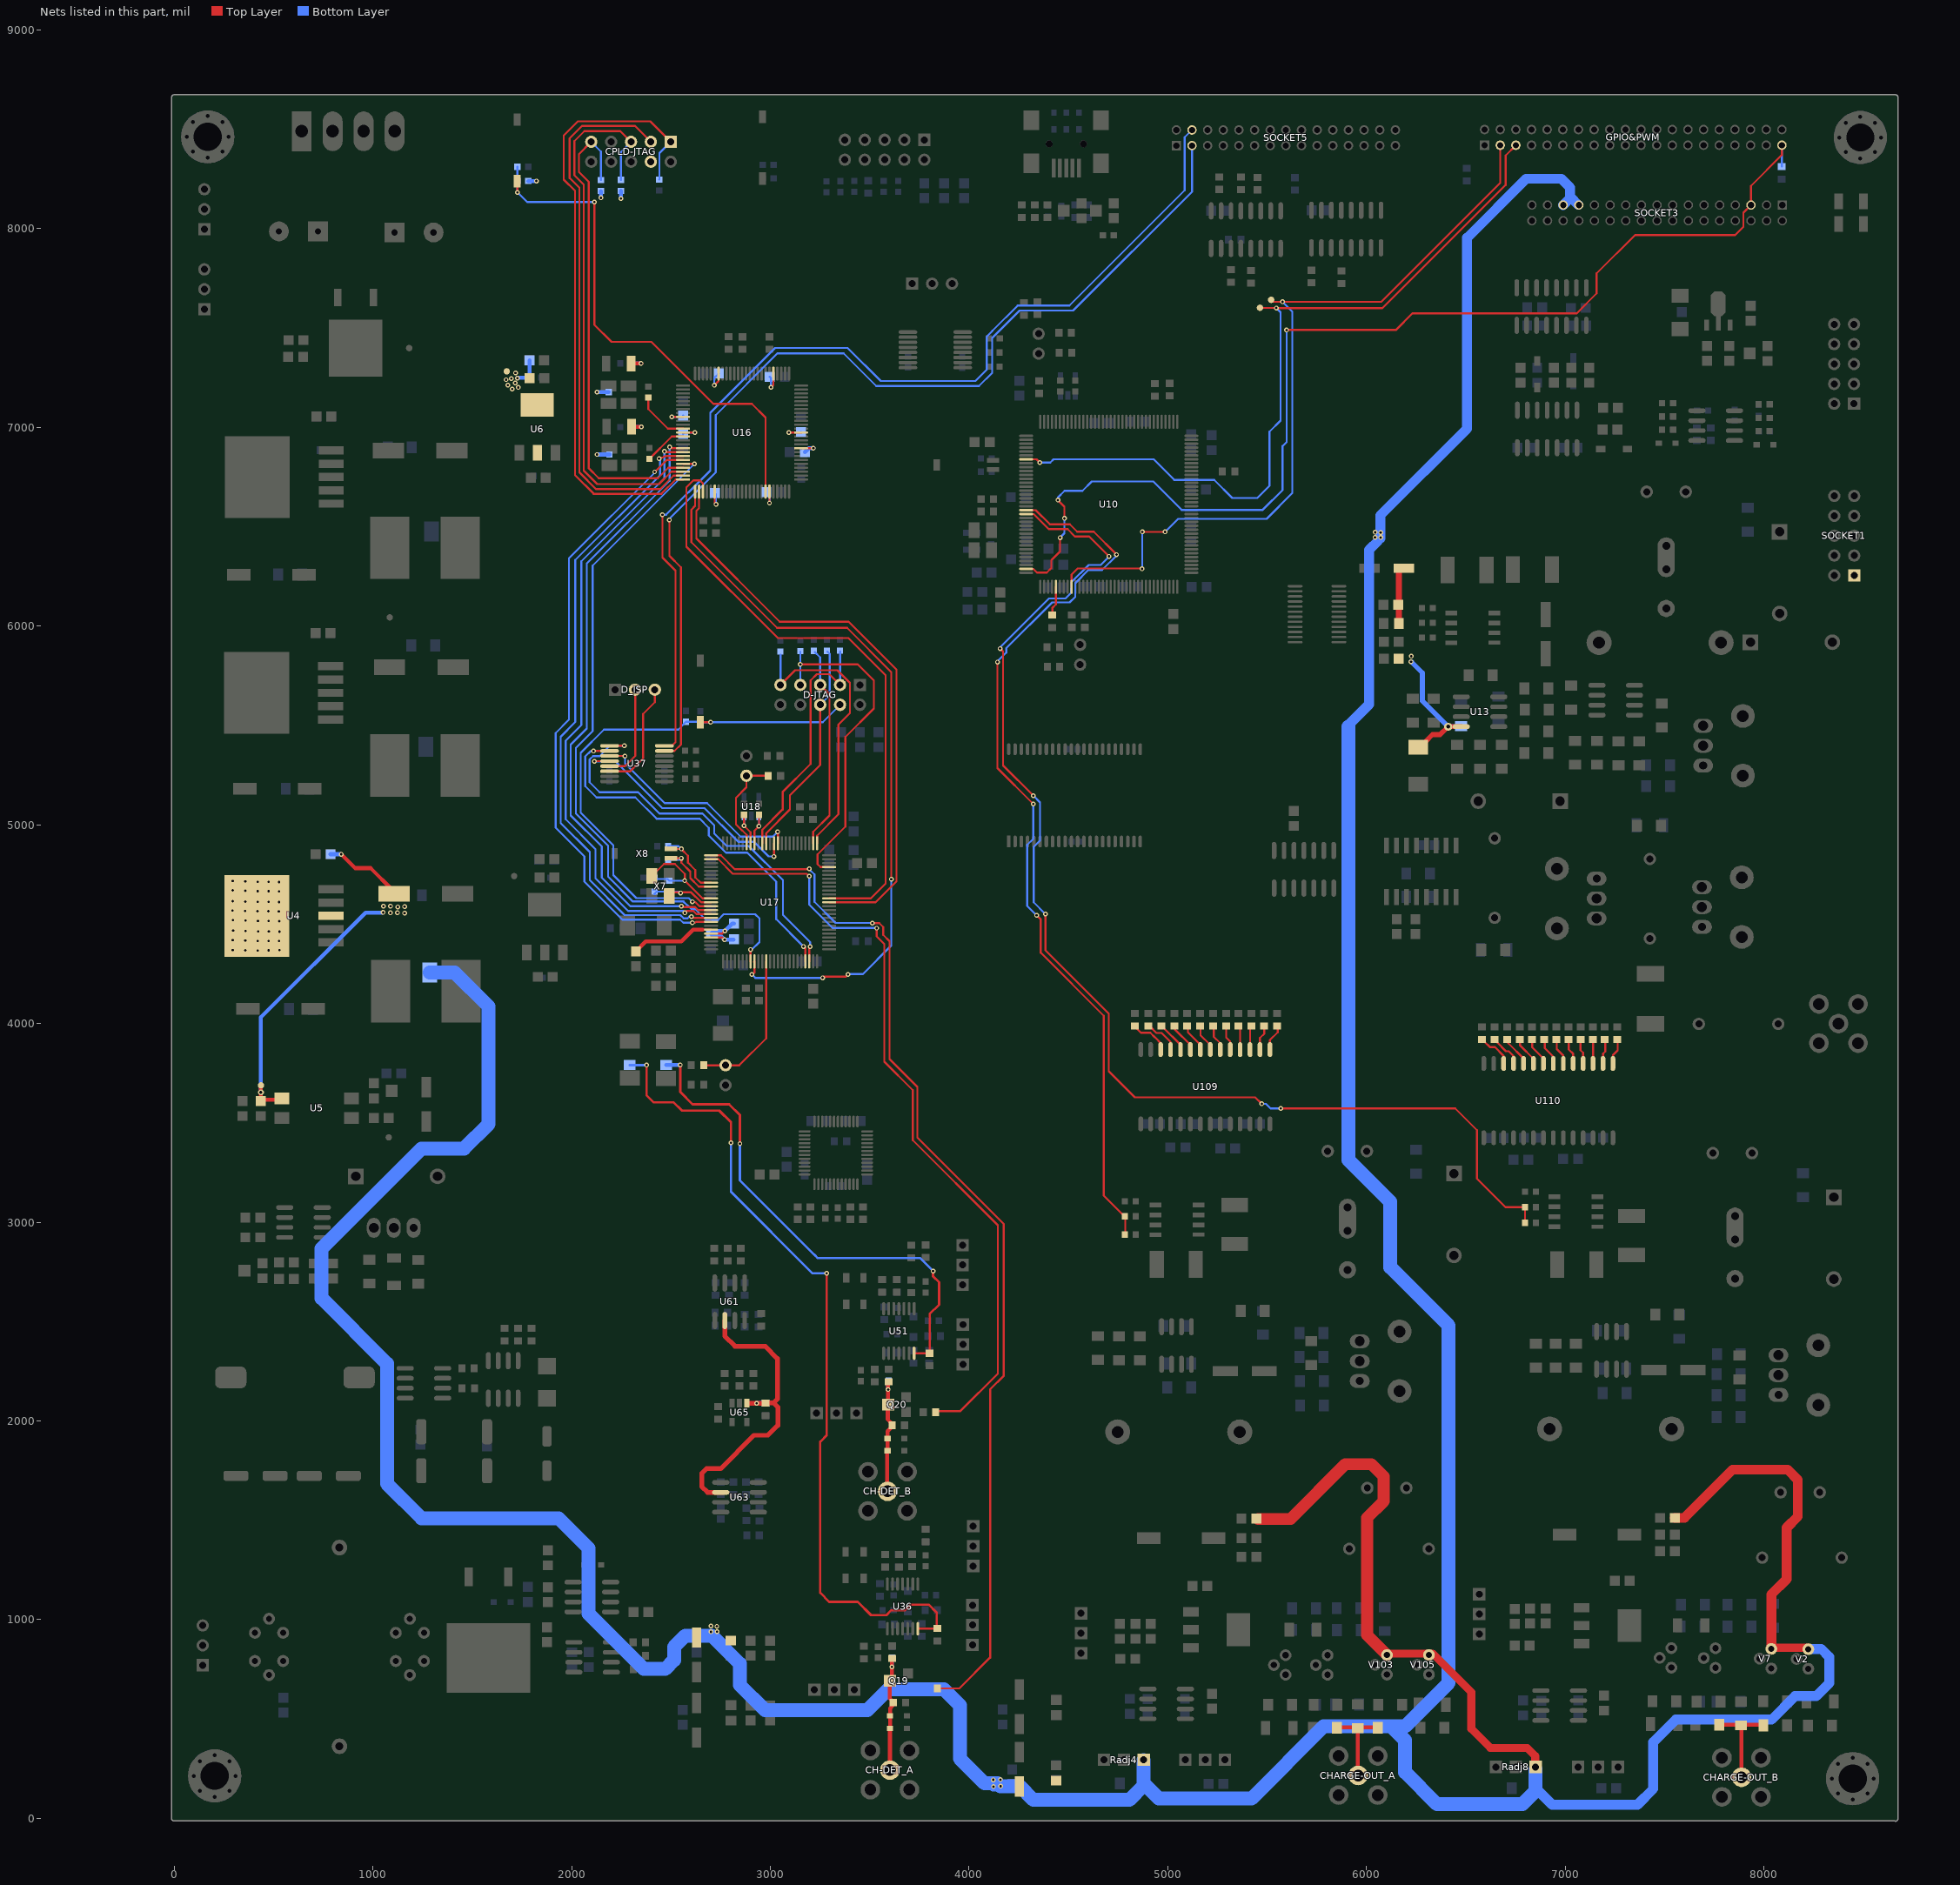
[diagram p0: the nets of this part, all layers, seen from the top]
# Altium PCB MISC82309.PcbDoc (part 5 of 14)
Units mil, origin at the board's own origin, x right, y up, seen from the top; angles counter-clockwise.
Board outline 8687.03 x 8687.86 mil, 4 copper layers (Top Layer, GND, POWER, Bottom Layer); 747 components, 583 nets, 2530 pads, 1834 vias.

## Via types
v1: diameter 24, hole 12, Top Layer to Bottom Layer, 1799 vias
v2: diameter 30, hole 15, Top Layer to Bottom Layer, 26 vias
v3: diameter 40, hole 20, Top Layer to Bottom Layer, 9 vias

## Nets (pads, with @x,y where several pads share a name; then routed paths per layer and width w, separated by ;. In a path a pad name is that pad's centre, name@x,y a point inside that pad or via, vN(x,y) a via of type N, cw(c..) or ccw(c..) an arc to the next point about the centre after c; other vN are vias at no path point) (continued)
-12V: C12.2 C13.2 C64.2 C65.2 C69.1 C156.1 C159.2 C174.2 C175.2 C278.1 D4.1 FB3.1 FB6.1 FB20.1 R4.1 R11.1 R45.1 R296.1 Radj4.3 Radj8.3 SOCKET3.27 SOCKET3.29 TP4.1 U4.3 U4.6 U5.3 V2.3 V7.3 V103.3 V105.3 | length 29056.6
  Top Layer w20: R11.1@437,3609.5 v2(437,3654) TP4.1@437,3689 ; R11.1@442,3616 U5.3@534.61,3616 ; v1(841,4852) 911,4782 989,4782 C12.2@1099,4672
  Top Layer w30: U5.3@534.61,3616 U5.3@542.8,3624.2 ; FB3.1@6163.39,6013 C64.2@6163.39,6286.61
  Top Layer w40: V103.3@6103,822.21 6110.32,829.53 6332.47,829.53 6527,635 6527,451 6623,355 6808,355 6849,314 Radj8.3@6849,266 ; Radj8.3@6850,263 Radj8.3@6850,266 ; V7.3@8037,853.21 8042.31,858.53 V2.3@8222.47,858.53
  Top Layer w50: R296.1@7551.5,1512 7599,1512 7842,1755 8119,1755 8170,1704 8170,1519 8114,1463 8114,1204 8037,1127 V7.3@8037,853.21
  Top Layer w60: R45.1@5455,1507 5618,1507 5894,1783 6024,1783 6086,1721 6086,1596 6003,1513 6003,922.21 V103.3@6103,822.21
  Bottom Layer w20: v2(437,3654) 437,4032 963,4558 v1@1049,4558 ; R4.1@787.5,4852 v1(841,4852) ; Radj4.3@4879,283 Radj4.3@4881,285 ; Radj8.3@6851,246 Radj8.3@6855,250
  Bottom Layer w50: v1@4122,161 v1@4159,161 ; Radj4.3@4881,285 Radj4.3@4881,296 ; 5917,5510 6013,5606 6013,6384 6059.5,6430.5 ; v1@6069,6471 6069,6557 6506,6994 6506,7954 6803,8251 6980,8251 7025,8206 7025,8154.36 SOCKET3.29@6989.64,8119 ; v1@6070,6441 v1@6070,6468 ; C278.1@6851,152 6934,69 7363,69 7443,149 7443,384 7556,497 8038,497 8156,615 8263,615 8329,681 8329,812 8288,853 V2.3@8232,853 ; Radj8.3@6851,246 Radj8.3@6851,259 Radj8.3@6851,263 ; 7030.64,8154.36 SOCKET3.27@7065,8120
  Bottom Layer w70: D4.1@1287,4257 1411,4257 1582,4086 1582,3494 1459,3371 1245,3371 742,2868 742,2618 1071,2289 1071,1684 1245,1510 1935,1510 2086,1359 2086,1030 2364,752 2471,752 2516,797 2516,863 2573,920 2705,920 2847,778 2847,671 2973,545 3489,545 3593,649 3874,649 3954,569 3954,301 4079,176 4143,176 ; v1(4159,162) 4255,162 4324,93 4806,93 4878,165 Radj4.3@4878,293 ; C69.1@4879,176 4955,100 5421,100 5784,463 6124,463 ; 5910,5493 5910,3313 6120,3103 6120,2773 6413,2480 6413,682 6194,463 6124,463 ; Radj8.3@6851,246 C278.1@6851,152 6851,138 6784,71 6355,71 6194,232 6194,393 6124,463
  other v1: 4123,160 4122,194 4158,195 2701,939 2732,940 2731,967 2701,968 421,4367 358,4368 475,4368 530,4369 295,4370 528,4415 421,4416 475,4416 358,4418 295,4420 530,4463 423,4464 477,4464 360,4466 297,4468 529,4515 422,4516 476,4516 359,4518 296,4520 1160,4556 1088,4557 1124,4558 1052,4559 527,4564 420,4565 474,4565 357,4567 294,4569 1125,4587 1160,4588 1089,4590 1053,4591 528,4611 421,4612 475,4612 358,4614 295,4616 528,4665 421,4666 475,4666 358,4668 295,4670 528,4712 421,4713 475,4713 358,4715 295,4717 6071,6446 6043,6447 6071,6471 6044,6472
-VCC: C423.1 C424.2 U61.6 U63.6 U65.1 | length 1590.4
  Top Layer w24: U63.6@2760,1641 2754,1641 U63.6@2750.51,1641 2684,1641 2654.5,1670.5 2654.5,1735.5 2679,1760 2750,1760 2918,1928 2988,1928 3038,1978 3038,2070 3018,2090 ; U61.6@2771,2505.51 2771,2427 2822,2376 2974,2376 3036,2314 3036,2110 3018,2092 3018,2090 ; U65.1@2882.4,2089.24 v1@2931.24,2089.24 ; v1(2931,2089) v1@2931.24,2089.24 ; C423.1@2978,2090 3018,2090 ; C423.1@2978,2091 2976.24,2089.24 v1@2931.24,2089.24
  Bottom Layer w24: v1(2931,2089) C424.2@2976,2089
AMP-12V: C53.1 D55.1 R91.2 U13.4 | length 672.8
  Top Layer w25: D55.1@6298,5420 6332,5454 6370,5454 6410,5494 v3(6411,5494) U13.4@6476.51,5494
  Bottom Layer w25: v1@6226,5820 6281,5765 6281,5624 v3(6411,5494) C53.1@6472,5494
  other v1: 6224,5821 6225,5848
ARM_PC5: GPIO&PWM.3 TP7.1 U10.45 | length 4034.9
  Top Layer w10: U10.45@4515.99,6197.65 4515.99,6258.99 4547,6290 4797,6290 ; 4803,6290 4797,6290 ; v1(4870,6288) 4868,6290 4797,6290 ; v1(4872,6474) v1(4986,6474) ; TP7.1@5520,7642 5530,7632 v1(5577,7632) 6074,7632 6672.74,8230.74 6672.74,8385 GPIO&PWM.3@6672.74,8420
  Bottom Layer w10: v1(4870,6288) 4872,6290 v1(4872,6474) ; v1(4986,6474) 5052,6540 5497,6540 5627,6670 5627,7582 v1(5577,7632)
ARM_PC8: GPIO&PWM.5 TP8.1 U10.7 | length 3976.5
  Top Layer w10: U10.7@4287.65,6839.38 4339.62,6839.38 v1(4356,6823) ; TP8.1@5473,7601 v1(5546,7601) 5547,7600 6080,7600 6700,8220 6700,8368.52 GPIO&PWM.5@6751.48,8420
  Bottom Layer w10: v1(4356,6823) 4408.62,6823 4425,6839.38 4929.62,6839.38 5033,6736 5234,6736 5325,6645 5450.94,6645 5512,6706.06 5512,6978 5568,7034 5568,7579 v1(5546,7601)
C_3V3: C20.2 C34.2 C75.2 C195.2 C196.2 C197.2 C198.2 C199.2 C200.2 C201.2 C202.2 C449.2 CPLD-JTAG.4 FB1.1 FB4.1 R16.1 R58.2 R100.1 R108.2 R232.2 R234.2 SOCKET1.1 TP6.1 U6.2 U6.4 U16.9 U16.13 U16.31 U16.45 U16.59 U16.63 U16.80 U16.94 | length 1540
  Top Layer w10: v1(2505,7053) 2506.48,7053 2506.74,7052.74 U16.9@2560.76,7052.74 ; U16.13@2560.76,6974 v1(2620,6974) ; v1(2718,7212) 2739.89,7233.89 U16.94@2739.89,7271.24 ; U16.31@2720.2,6676.76 2720.2,6619.8 v1(2727,6613) ; v1(2995.8,6619.8) U16.45@2995.8,6676.76 ; v1(3004,7202) 3015.48,7213.48 U16.80@3015.48,7271.24 ; v1(3093,6974) U16.63@3155.24,6974 ; U16.59@3155.24,6895.26 v1(3216.74,6895.26)
  Top Layer w20: FB1.1@2299.99,7322 v1(2350,7322) ; FB4.1@2301.99,7003 v1(2351,7003)
  Bottom Layer w10: v1@2512,7053 2554.5,7053 C199.2@2561,7059.5 ; C195.2@2561,6967.5 2567.5,6974 v1@2618,6974 ; v1@2718,7215 2718,7248.5 C197.2@2740.5,7271 ; C196.2@2720.5,6669 2726,6663.5 v1@2726,6616 ; v1@2996,6623 2996.5,6623.5 C200.2@2996.5,6676 ; C201.2@2997.5,7254 3004,7247.5 v1@3004,7206 ; v1@3095,6975 3151.5,6975 C202.2@3154,6977.5 ; C198.2@3154,6889.5 C198.2@3158.5,6894
  Bottom Layer w20: v1@1728,7249 1786,7249 1790,7253 1788.5,7254.5 R16.1@1788.5,7338 ; R100.1@1782.5,8240 v1(1823,8240) ; v1(2128.5,6863.5) R108.2@2191,6863.5 ; v1(2128.5,7177.5) R58.2@2187,7177.5 ; v1(2148,8155) R234.2@2148,8189.5 ; v1(2248,8152) R232.2@2248,8190.5 ; C34.2@2299.5,7322 v1@2347,7322 ; C75.2@2300.5,7002 2350,7002 v1(2351,7003) ; C198.2@3173.5,6876 3193.5,6896 v1@3217,6896
  other v1: 1701,7193 1732,7201 1679,7213 1717,7223 1671,7240 1697,7246 1727,7248 1718,7274
CH-DET_A: R199.2 R207.1 U36.7 | length 4187.7
  Top Layer w12: v1(2377,3791) 2377,3639 2412,3604 2513,3604 2555,3562 2743,3562 2802,3503 v1(2802,3400) ; v1(3284,2743) 3284,1929 3251,1896 3251,1135 3296,1090 3440,1090 3507,1023 3585,1023 3609.5,1047.5 3677.5,1047.5 3706,1076 3797,1076 3837,1036 R199.2@3837,961 ; U36.7@3742.77,954.8 3835.8,954.8 R199.2@3840,959
  Bottom Layer w12: R207.1@2292,3791 v1(2377,3791) ; v1@2802,3399 v1(2802,3400) 2802,3153 3212,2743 v1(3284,2743)
CH-DET_B: R110.1 R339.2 U51.7 | length 2580.3
  Top Layer w12: v1(2547,3792) 2547,3656 2609,3594 2793,3594 2847,3540 v1(2847,3395) ; U51.7@3723.77,2340.8 R339.2@3802,2340.8 ; R339.2@3802,2340.5 R339.2@3802,2340.8 ; R339.2@3807,2337 3803.2,2340.8 R339.2@3802,2340.8 ; v1(3819,2754) 3819,2728 3849,2698 3849,2585 3802,2538 R339.2@3802,2340.8
  Bottom Layer w12: v1(2847,3395) 2847,3351 2847,3211 3226,2832 ; 3223,2836 3239.5,2819.5 3754.5,2819.5 v1@3818,2756 ; v1@3816.5,2756.5 v1(3819,2754)
  Bottom Layer w20: R110.1@2476,3791 2477,3792 v1@2545,3792
CH-DETECT-IN_A: C165.2 CH-DET_A.1 D25.1 D26.2 Q19.3 R186.1 R545.2 | length 600.5
  Top Layer w20: CH-DET_A.1@3602,243 3602,436 3603,437 3603,555 3619,571 3619,586 3601,604 3601,672 Q19.3@3602,673 ; Q19.3@3602,692.5 3612,702.5 v1(3612,762) R186.1@3612,802
  Bottom Layer w20: v1@3612,767 3612,807.5 C165.2@3613,808.5
CH-DETECT-IN_B: C288.2 CH-DET_B.1 D46.2 D47.1 Q20.3 R322.1 R546.2 | length 601.9
  Top Layer w20: CH-DET_B.1@3587,1644 3588,1645 3588,1849 3589.68,1850.68 D47.1@3589.68,1912 3589.68,1948.68 3610,1969 3610,1988 3591,2007 Q20.3@3591,2064 ; Q20.3@3593,2082.5 3593,2196 R322.1@3597,2200
  Bottom Layer w20: v1(3593,2158) 3593,2200.5 C288.2@3595,2202.5
CH_A: R378.2 U17.1 | length 5378.3
  Top Layer w10: U17.1@2701.76,4846.22 2751.78,4846.22 2821,4777 3194,4777 v1(3196,4779) ; v1(3513,4505) 3548,4505 3568,4485 3568,4446 3600,4414 3600,3821 3740,3681 3740,3426 4175,2991 4175,2228 4106,2159 4106,809 3951,654 R378.2@3848,654
  Bottom Layer w10: v1(3196,4779) 3196,4775.94 3222,4749.94 3222,4612 3328,4506 3512,4506 v1(3513,4505)
CH_B: R379.2 U17.2 | length 3935.7
  Top Layer w10: U17.2@2701.76,4826.54 2738.46,4826.54 2811,4754 3183,4754 3195,4742 v1(3196,4742) ; v1(3535,4480) 3535,4439 3574,4400 3574,3808 3717,3665 3717,3413 4145,2985 4145,2238 3957,2050 R379.2@3843,2050
  Bottom Layer w10: v1(3196,4742) 3196,4598 3313,4481 3534,4481 v1(3535,4480)
CH_PHASE1: U16.17 U17.15 | length 3129.6
  Top Layer w10: v1(2493,6901) 2493,6900 2498,6895 2498.26,6895.26 U16.17@2560.76,6895.26 ; v1(2553,4590) 2553,4585 2554,4586 2621,4586 2636.37,4570.63 U17.15@2701.76,4570.63
  Bottom Layer w10: v1(2493,6901) 2493,6731 2077,6315 2077,5485 1996,5404 1996,5047 2152,4891 2152,4734 2296,4590 v1(2553,4590)
CH_PHASE2: U16.18 U17.16 | length 3156.2
  Top Layer w10: v1@2471.57,6875.57 U16.18@2560.76,6875.57 ; 2579,4566 2613,4566 2628.06,4550.94 U17.16@2701.76,4550.94
  Bottom Layer w10: v1(2467,6879) 2467,6744 2049,6326 2049,5502 1970,5423 1970,5028 2120.69,4877.31 2120.69,4730.31 2285,4566 2561,4566 v1(2570,4557)
CH_PHASE3: U16.19 U17.17 | length 3186.1
  Top Layer w10: v1(2440,6843) 2438,6843 2437,6844 2441,6848 2460.96,6848 2467.96,6855 2476.94,6855 ; 2477.83,6855.89 U16.19@2560.76,6855.89 ; v1@2612.74,4531.26 U17.17@2701.76,4531.26
  Bottom Layer w10: v1@2445,6836 2445,6759 2019,6333 2019,5517 1945,5443 1945,5009 2091.5,4862.5 2091.5,4721.5 2266.97,4546.03 2547.03,4546.03 2564.06,4529 2583,4529 v1@2592,4538
  other v1: 2603,4538
CH_PHASE4: U16.20 U17.18 | length 3209.2
  Top Layer w10: v1@2419,6776 2479.2,6836.2 U16.20@2560.76,6836.2 ; 2622,4507 2626.57,4511.57 U17.18@2701.76,4511.57
  Bottom Layer w10: v1@2423.5,6777.5 1987,6341 1987,5529 1920,5462 1920,4986 2065,4841 2065,4714 2256,4523 2546.02,4523 2562.02,4507 v1(2608,4507)
  other v1: 2418,6776
CH_PHASE5: U16.21 U17.33 | length 3562.8
  Top Layer w10: U16.21@2560.76,6816.52 v1(2618.48,6816.52) ; U17.33@2900.57,4312.76 v1(2900.57,4372.57) ; U17.33@2901.48,4312.76 U17.33@2901.48,4318.02
  Bottom Layer w10: 2581.94,4595 2562.94,4614 2309,4614 2184,4739 2184,4895 2022,5057 2022,5387 2106.5,5471.5 2106.5,6304.5 2618,6816 v1@2618.48,6816 ; 2584,4595 2604,4575 2623,4575 2677,4521 2736,4521 2765,4550 2924,4550 2945,4529 2945,4410.52 2907.05,4372.57 v1(2900.57,4372.57)
CH_PHASE6: U16.26 U17.34 | length 3745.1
  Top Layer w10: U16.26@2621.78,6676.76 2621.78,6604.78 2603,6586 2603,6422 3034,5991 3386,5991 3609,5768 v1(3609,4726) ; v1@2913,4249 2920.26,4256.26 U17.34@2920.26,4312.76 U17.34@2918.48,4310.98 ; v1@3269,4236 3380,4236 v1(3391,4247)
  Bottom Layer w10: v1@2914,4246 2914,4241 2925,4230 v1(3263,4230) ; v1@3393,4249 3466,4249 3609,4392 v1(3609,4726)
  other v1: 2907,4247
CH_PHASE7: U16.27 U17.63 | length 2970
  Top Layer w10: U16.27@2641.46,6676.76 2641.46,6593.46 2628,6580 2628,6441 3047,6022 3394,6022 3635,5781 3635,4715 3530,4610 U17.63@3296.24,4610
CH_PHASE8: U16.28 U17.64 | length 3076.6
  Top Layer w10: U16.28@2661.15,6676.76 2661.15,6718 2646.15,6733 2613,6733 2578,6698 2578,6400 3038,5940 3393,5940 3580,5753 3580,4704 3505.68,4629.68 U17.64@3296.24,4629.68
CHARGE-CTRL_A: R151.2 R312.2 U10.20 | length 4596.2
  Top Layer w10: v1(4143,5819) 4143,5285 v1(4323,5105) ; U10.20@4287.65,6583.47 4335.53,6583.47 4407,6512 4507,6512 4544,6475 4628,6475 v1@4742.5,6360.5 ; v1(4340,4545) 4361,4524 4361,4356 4678,4039 4678,3134 4786,3026 R151.2@4786,2939
  Bottom Layer w10: v1@4143,5823 4187,5867 4187,5888 4418,6119 4506,6119 4534,6147 4534,6216 4600,6282 4668.94,6282 4742,6355.06 v1(4742,6360) v1@4741.5,6359.5 ; v1(4323,5105) 4323,4929 4293,4899 4293,4592 v1(4340,4545)
CHARGE-CTRL_B: R343.2 R344.2 U10.21 | length 6265.2
  Top Layer w10: v1(4156,5887) 4171,5872 4171,5299 v1(4323,5147) ; U10.21@4287.65,6563.79 4325.21,6563.79 4401,6488 4495.79,6488 4532.79,6451 4604,6451 v1(4704,6351) ; v1(4384,4551) 4384,4369 4703,4050 4703,3760 4834,3629 5440,3629 v1(5473,3596) ; v1(5569,3573) 6446,3573 6556,3463 6556,3219 6699,3076 R344.2@6797,3076 ; R344.2@6796,3077 R344.2@6797,3076 ; R343.2@6797.5,2997 6797.5,3075.5 R344.2@6797,3076 ; R344.2@6797.5,3076 R344.2@6797,3076
  Bottom Layer w10: v1(4156,5887) 4153,5890 4402,6139 4485,6139 4514,6168 4514,6220.04 4601.96,6308 4663,6308 v1@4704,6349 ; v1(4323,5147) 4357,5113 4357,4921 4325,4889 4325,4610 v1(4384,4551) ; v1(4704,6351) v1@4704,6349 ; v1@4705,6350 v1@4704,6349 ; v1(5473,3596) 5494,3596 5517,3573 v1(5569,3573)
CHARGE_OUT_A: CHARGE-OUT_A.1 R152.1 R202.2 R203.2 | length 426.1
  Top Layer w20: R203.2@5852,461 5854,459 6054,459 R152.1@6057,456 ; CHARGE-OUT_A.1@5956,235 R202.2@5956,454
CHARGE_OUT_B: CHARGE-OUT_B.1 R302.2 R303.2 R304.1 | length 478
  Top Layer w20: R303.2@7774,472 R304.1@7997,472 ; CHARGE-OUT_B.1@7887,207 R302.2@7887,462
CLK0: R59.1 U16.12 | length 274
  Top Layer w10: R59.1@2386,7150.5 2386,7092 2484.32,6993.68 U16.12@2560.76,6993.68
CLK1: R109.1 U16.14 | length 215.5
  Top Layer w10: R109.1@2392,6841.5 2504.81,6954.31 U16.14@2560.76,6954.31
COUNT-RESET: GPIO&PWM.39 R404.2 SOCKET3.5 U10.35 | length 5789.4
  Top Layer w10: U10.35@4287.65,6288.2 4322.81,6288.2 4342.01,6269 4391,6269 4414,6292 4414,6332 4458,6376 v1(4458,6445) ; v1(4447,6634) 4480,6601 v1(4480,6542) ; v1(5598,7490) 6147,7490 6231,7574 7058,7574 7158,7674 7158,7775 7351,7968 7855,7968 7896,8009 7896,8080.48 SOCKET3.5@7934.52,8119 7934.52,8215.52 8090.06,8371.06 GPIO&PWM.39@8090.06,8420
  Bottom Layer w10: v1(4447,6634) 4447,6647 4481,6681 4571,6681 4618,6728 4927,6728 5070,6585 5478,6585 5578,6685 5578,6906 5598,6926 v1(5598,7490) ; v1(4458,6445) 4480,6467 v1(4480,6542) ; R404.2@8090,8312.5 8090,8419.94 GPIO&PWM.39@8090.06,8420
CPLD_RST: C244.2 CPLD_REST.2 R100.2 U16.44 | length 2635.1
  Top Layer w10: CPLD_REST.2@1727,8239 1727,8183 v1(1727.5,8182.5) ; v1(2115,8134) 2115,7516 2201,7430 2402,7430 2713.94,7118.06 2907.06,7118.06 2976.11,7049 U16.44@2976.11,6676.76
  Bottom Layer w10: v1@1727.5,8176.5 1734.5,8176.5 1777,8134 v1(2115,8134) ; v1(1727.5,8182.5) R100.2@1727.5,8240 C244.2@1727.5,8311
CPLD_TCK: CPLD-JTAG.1 R294.2 U16.25 | length 3169.2
  Top Layer w10: CPLD-JTAG.1@2499,8437 2396,8540 2032,8540 1961,8469 1961,8247 2017,8191 2017,6760 2111,6666 2452,6666 2523.78,6737.78 U16.25@2560.76,6737.78
  Bottom Layer w10: R294.2@2441,8246.5 2442,8247.5 2442,8380 CPLD-JTAG.1@2499,8437
CPLD_TDI: CPLD-JTAG.9 R234.1 U16.22 | length 2418.5
  Top Layer w10: CPLD-JTAG.9@2099,8437 2037,8375 2037,8285 2087,8235 2087,6794 2137,6744 2434,6744 2486.83,6796.83 U16.22@2560.76,6796.83
  Bottom Layer w10: CPLD-JTAG.9@2099,8437 2148,8388 R234.1@2148,8244.5
CPLD_TDO: CPLD-JTAG.3 U16.24 | length 2753.6
  Top Layer w10: CPLD-JTAG.3@2399,8437 2319,8517 2052,8517 1990,8455 1990,8255 2039,8206 2039,6774 2123,6690 2446,6690 2513.46,6757.46 U16.24@2560.76,6757.46
CPLD_TMS: CPLD-JTAG.5 R232.1 U16.23 | length 2771.8
  Top Layer w10: CPLD-JTAG.5@2299,8437 2245,8491 2064,8491 2014,8441 2014,8269 2061,8222 2061,6783 2129,6715 2440,6715 2502.15,6777.15 U16.23@2560.76,6777.15
  Bottom Layer w10: R232.1@2248,8245.5 2248,8386 CPLD-JTAG.5@2299,8437
D_A0: R547.1 U109.12 | length 190.3
  Top Layer w10: R547.1@4840,3979 4865.5,3953.5 4912.5,3953.5 4935,3931 4939,3927 U109.12@4964,3902 ; U109.12@4964,3869.01 U109.12@4964,3902 ; U109.12@4965,3901 U109.12@4964,3902
D_A1: R548.1 U109.11 | length 175.9
  Top Layer w10: R548.1@4911,3985 4943,3953 4969,3953 5014,3908 U109.11@5014,3869.01 ; R548.1@4912,3979 R548.1@4912,3981
D_A2: R549.1 U109.10 | length 147
  Top Layer w10: R549.1@4977,3980 5064,3893 U109.10@5064,3869.01
D_A3: R550.1 U109.9 | length 155.3
  Top Layer w10: R550.1@5036,3992 5036,3970 5114,3892 U109.9@5114,3869.01
D_A4: R525.1 U109.8 | length 140.1
  Top Layer w10: R525.1@5101,3983 5101,3956 5164,3893 U109.8@5164,3869.01
D_A5: R526.1 U109.7 | length 134.3
  Top Layer w10: R526.1@5165,3983 5165,3941 5214,3892 U109.7@5214,3869.01
D_A6: R527.1 U109.6 | length 131.7
  Top Layer w10: R527.1@5231,3987 5231,3934 5264,3901 U109.6@5264,3869.01
D_A7: R528.1 U109.5 | length 125.3
  Top Layer w10: R528.1@5294,3986 5294,3930 5314,3910 U109.5@5314,3869.01
D_A8: R529.1 U109.4 | length 118.1
  Top Layer w10: R529.1@5359,3985 5364,3980 U109.4@5364,3869.01
D_A9: R530.1 U109.3 | length 117.4
  Top Layer w10: R530.1@5413,3986 5414,3985 U109.3@5414,3869.01
D_A10: R531.1 U109.2 | length 127.1
  Top Layer w10: U109.2@5464,3869.01 5464,3927 5486,3949 R531.1@5486,3987
D_A11: R532.1 U109.1 | length 134.1
  Top Layer w10: U109.1@5514,3869.01 5514,3917 5553,3956 R532.1@5553,3987
D_AGND: R222.1 U17.20 | length 433.1
  Top Layer w11: 2649.2,4472.2 2659.52,4472.2 U17.20@2701.76,4472.2
  Top Layer w20: R222.1@2324,4363.5 2373.5,4413 2552,4413 2611.2,4472.2 2659.52,4472.2
D_B0: R533.1 U110.12 | length 170.8
  Top Layer w10: R533.1@6593,3913 6593,3909 6620,3882 6645,3882 6690,3837 U110.12@6690,3799.01 U110.12@6690,3801
D_B1: R534.1 U110.11 | length 152
  Top Layer w10: R534.1@6656,3908 6656,3906 6701,3861 6715,3861 6740,3836 U110.11@6740,3799.01
D_B2: R535.1 U110.10 | length 157.4
  Top Layer w10: R535.1@6713,3922 6713,3901 6793,3821 6793,3802.01 U110.10@6790,3799.01
D_B3: R536.1 U110.9 | length 140.7
  Top Layer w10: R536.1@6773,3912 6773,3889 6840,3822 U110.9@6840,3799.01
D_B4: R537.1 U110.8 | length 142.2
  Top Layer w10: R537.1@6834,3918 6834,3880 6890,3824 U110.8@6890,3799.01
D_B5: R538.1 U110.7 | length 136.8
  Top Layer w10: R538.1@6897,3918 6897,3876 6940,3833 U110.7@6940,3799.01
D_B6: R539.1 U110.6 | length 128.7
  Top Layer w10: R539.1@6957,3914 6957,3872 6990,3839 U110.6@6990,3799.01
D_B7: R540.1 U110.5 | length 127.5
  Top Layer w10: R540.1@7017,3917 7017,3870 7040,3847 U110.5@7040,3799.01
D_B8: R541.1 U110.4 | length 122.4
  Top Layer w10: R541.1@7077,3916 7077,3866 7090,3853 U110.4@7090,3799.01
D_B9: R542.1 U110.3 | length 121.4
  Top Layer w10: R542.1@7139,3920 7140,3919 U110.3@7140,3799.01
D_B10: R543.1 U110.2 | length 121.5
  Top Layer w10: U110.2@7190,3799.01 7190,3848 7201,3859 R543.1@7201,3916
D_B11: R544.1 U110.1 | length 123.9
  Top Layer w10: U110.1@7240,3799.01 7240,3841 7264,3865 R544.1@7264,3913
D_BOOT0: D_BOOT0.2 R61.1 U17.94 | length 493.1
  Top Layer w10: U17.94@2880.89,4907.24 2880.89,4949.11 2859,4971 2858.06,4971 2827,5002.06 2827,5136 2880,5189 D_BOOT0.2@2880,5247 R61.1@2988.5,5247
D_BOOT1: D_BOOT1.2 R62.1 U17.37 | length 757.7
  Top Layer w10: R62.1@2665.5,3791 2666.5,3790 D_BOOT1.2@2775,3790 2844,3790 2979.32,3925.32 U17.37@2979.32,4312.76
D_ISP_RX: D_ISP.2 U37.13 | length 485.1
  Top Layer w10: U37.13@2191.2,5295.2 2269.2,5295.2 2321,5347 2321,5678 D_ISP.2@2319,5680
D_ISP_TX: D_ISP.3 U37.14 | length 565.9
  Top Layer w10: U37.14@2191.2,5269.61 2295.61,5269.61 2360,5334 2360,5558 2419,5617 D_ISP.3@2419,5680
D_JNTRST: D-JTAG.3 R592.1 U17.90 | length 1273.6
  Top Layer w10: U17.90@2959.63,4907.24 2959.63,4974.63 3062,5077 3062,5098 3062,5165 3203,5306 3203,5727 3234,5758 3297,5758 D-JTAG.3@3351,5704
  Bottom Layer w10: D-JTAG.3@3351,5704 3351,5871 R592.1@3353,5873
D_JTCK: D-JTAG.9 R595.2 U17.76 | length 1436.1
  Top Layer w10: D-JTAG.9@3051,5704 3125,5778 3232,5778 3337.81,5778 3401,5714.81 3401,5562 3343,5504 3343,5053 3235.22,4945.22 U17.76@3235.22,4907.24
  Bottom Layer w10: D-JTAG.9@3051,5704 R595.2@3051,5857
D_JTDI: D-JTAG.5 R593.1 U17.77 | length 1028
  Top Layer w10: U17.77@3215.54,4907.24 3215.54,4964.54 3298,5047 3298,5657 D-JTAG.5@3251,5704
  Bottom Layer w10: R593.1@3223,5870 3251,5842 D-JTAG.5@3251,5704
D_JTDO: D-JTAG.6 R596.2 U17.89 | length 1100.7
  Top Layer w10: U17.89@2979.32,4907.24 2979.32,4957.32 3099,5077 3099,5102 3099,5149 3251,5301 D-JTAG.6@3251,5604
  Bottom Layer w10: D-JTAG.6@3251,5604 3299,5652 3299,5860 R596.2@3288,5871
D_JTMS: D-JTAG.7 R594.1 U17.72 | length 1692.6
  Top Layer w10: v1(3151,5808) 3439,5808 3521,5726 3521,5585 3378,5442 3378,4991 3238,4851 3238,4802 3252.83,4787.17 U17.72@3296.24,4787.17
  Bottom Layer w10: D-JTAG.7@3151,5704 3151,5773 ; 3151,5788 3151,5773 ; R594.1@3151,5872 v1(3151,5808) 3151,5773
D_NRST: C74.2 D-JTAG.4 D_REST.1 R113.2 U17.14 | length 2697.2
  Top Layer w10: v1@2608,4611 2623,4611 2643.68,4590.32 U17.14@2701.76,4590.32 ; D_REST.1@2648,5516 v1@2699.5,5516
  Bottom Layer w10: v1(2608,4613) 2590,4631 2326,4631 2210,4747 2210,4897 2046,5061 2046,5362 2163.25,5479.25 2536.75,5479.25 C74.2@2576,5518.5 2646,5518.5 R113.2@2648,5516.5 v1(2700,5516.5) 3263.5,5516.5 D-JTAG.4@3351,5604
D_OSC32_IN: C84.2 U17.8 X8.1 | length 385.5
  Top Layer w10: X8.1@2500,4878.62 v1(2553,4878.62) v1@2554,4878.62 ; v1@2554,4876 2585.5,4844.5 ; 2585,4844 2585,4810 2623,4772 2623,4735 2649.57,4708.43 U17.8@2701.76,4708.43
  Bottom Layer w10: C84.2@2486.5,4893 2538.62,4893 v1(2553,4878.62)
D_OSC32_OUT: C85.2 U17.9 X8.4 | length 365.1
  Top Layer w10: X8.4@2502.38,4829 X8.4@2500,4831.38 v1@2553,4831.38 ; v1@2553,4831 2553,4809 2597,4765 2597,4732 2640.26,4688.74 U17.9@2701.76,4688.74
  Bottom Layer w10: C85.2@2486.5,4824 2544,4824 v1(2552,4832)
D_OSC_IN: C80.2 R114.1 U17.12 X7.1 | length 571.2
  Top Layer w10: X7.1@2404,4742 2465,4803 2520,4803 2570,4753 2570,4719 2659.32,4629.68 U17.12@2701.76,4629.68
  Bottom Layer w10: C80.2@2415.5,4727 2482.5,4727 R114.1@2491,4718.5 v1@2568.5,4718.5
  other v1: 2569,4719
D_OSC_OUT: C81.2 R114.2 U17.13 X7.3 | length 380.7
  Top Layer w10: X7.3@2490.61,4642 2508.61,4660 2602,4660 2652,4610 U17.13@2701.76,4610
  Bottom Layer w10: C81.2@2415.5,4651 2428,4663.5 2542.5,4663.5 v1(2549,4657)
D_OUT: R558.1 U10.41 | length 140.2
  Top Layer w10: R558.1@4419,6065 4419,6091 4437.25,6109.25 U10.41@4437.25,6197.65
D_RS232_RXD: SOCKET5.4 U37.8 | length 5264.8
  Top Layer w10: v1(2457,6560) 2457,6345 2523,6279 2523,5416 2504.57,5397.57 U37.8@2466.8,5397.57
  Bottom Layer w10: v1@2457,6561 2476,6561 2698,6783 2698,7074 3024,7400 3389,7400 3556,7233 4032,7233 4089,7290 4089,7457 4114,7482 4118,7486 4245,7613 4505,7613 5085,8193 5085,8460 SOCKET5.4@5121.74,8496.74
D_RS232_TXD: SOCKET5.3 U37.7 | length 5201.4
  Top Layer w10: U37.7@2466.8,5371.98 2517.98,5371.98 2550,5404 2550,6296 2492,6354 v1@2492,6528
  Bottom Layer w10: v1@2492,6535 2492,6541 2725,6774 2725,7062 3035,7372 3369,7372 3533,7208 4050,7208 4116,7274 4116,7450 4254,7588 4524,7588 5121.74,8185.74 SOCKET5.3@5121.74,8418
  other v1: 2492,6534
D_SCL: R111.2 U17.92 U18.1 | length 204.7
  Top Layer w10: U17.92@2920.26,4907.24 2920.26,4970.26 v1(2943,4993) R111.2@2943,5050.5
  Bottom Layer w10: U18.1@2942.4,5044.76 2943,5044.16 v1(2943,4993)
D_SDA: R112.2 U17.93 U18.3 | length 206.7
  Top Layer w10: R112.2@2868,5050.5 v1(2868,4995) 2900.57,4962.43 U17.93@2900.57,4907.24
  Bottom Layer w10: U18.3@2867.6,5044.76 2867.6,4995.4 v1(2868,4995)
D_USART2_RX: U17.87 U37.12 | length 1244.5
  Top Layer w10: v1(2115,5319) 2116.8,5320.8 U37.12@2191.2,5320.8 ; v1(3018,4841) 3018.68,4841.68 U17.87@3018.68,4907.24
  Bottom Layer w10: v1(2115,5319) 2221,5319 2456,5084 2669,5084 2838,4915 2917,4915 2991,4841 v1(3018,4841)
D_USART2_TX: U17.86 U37.11 | length 1104.2
  Top Layer w10: U37.11@2191.2,5346.39 2268.61,5346.39 v1(2269,5346) ; v1(3037,4965) 3038.37,4963.63 U17.86@3038.37,4907.24
  Bottom Layer w10: v1(2269,5346) 2269,5308 2468,5109 2682,5109 2850,4941 3013,4941 v1(3037,4965)
D_USART3_RX: U17.48 U37.9 | length 2060.5
  Top Layer w10: U37.9@2191.2,5397.57 2264.57,5397.57 v1(2265,5398) ; U17.48@3195.85,4312.76 3195.85,4381.85 v1(3201,4387)
  Bottom Layer w10: v1(2265,5398) 2193,5398 2141,5346 2108.06,5346 2091,5328.94 2091,5214 2141,5164 2335,5164 2442,5057 2659,5057 2718,4998 2718,4956 2780,4894 2891,4894 3063.5,4721.5 3063.5,4546.5 3201,4409 v1(3201,4387)
D_USART3_TX: U17.47 U37.10 | length 1925.7
  Top Layer w10: v1@2110.98,5371.98 U37.10@2191.2,5371.98 ; v1(3167,4388) 3176.17,4378.83 U17.47@3176.17,4312.76
  Bottom Layer w10: v1(2110,5371) 2096,5371 2069,5344 2069,5195 2126,5138 2321,5138 2428,5031 2644,5031 2691,4984 2691,4946 2777,4860 2884,4860 3029.5,4714.5 3029.5,4525.5 v1(3167,4388)
D_VDDA: C72.2 C73.2 R225.2 U17.21 U17.22 | length 413.4
  Top Layer w11: U17.22@2701.76,4432.83 2759.17,4432.83 v1(2770,4422) ; U17.21@2701.76,4452.52 2757.52,4452.52 v1(2771,4466)
  Bottom Layer w11: C72.2@2814.51,4422 C72.2@2817.5,4425
  Bottom Layer w20: C72.2@2814.51,4422 v1(2770,4422) 2752,4440 2713.5,4440 R225.2@2702,4451.5 2716.5,4466 v1(2771,4466) 2808,4503 C73.2@2817.5,4503